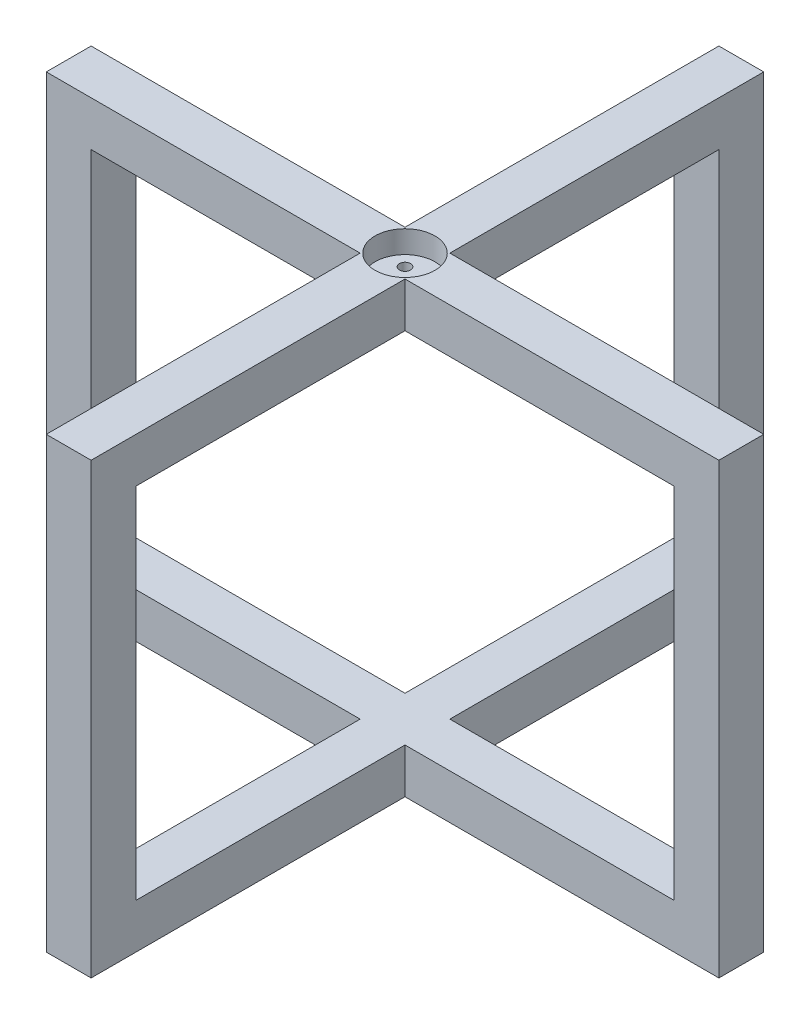
SolidWorks part; units mm, degrees
ref_plane "Front Plane" through (0, 0, 0) normal (0, 0, 1) x (1, 0, 0)
ref_plane "Top Plane" through (0, 0, 0) normal (0, 1, 0) x (1, 0, 0)
ref_plane "Right Plane" through (0, 0, 0) normal (1, 0, 0) x (0, 0, -1)
sketch "Sketch1" plane through (0, 0, 0) normal (0, 0, 1) x (1, 0, 0)
  line L0 (-450, 300) -> (450, 300)
  line L1 (-390, -240) -> (390, -240)
  line L2 (-390, -240) -> (-390, 240)
  line L3 (-390, 240) -> (390, 240)
  line L4 (390, -240) -> (390, 240)
  line L5 (0, 240) -> (0, -240) construction
  line L6 (-390, 0) -> (390, 0) construction
  line L7 (450, -300) -> (450, 300)
  line L8 (-450, -300) -> (450, -300)
  line L9 (-450, -300) -> (-450, 300)
  point P0 (0, 0)
  dimension "D2" = 900
  dimension "D3" = 600
  dimension "D1" = 60
extrude "Boss-Extrude1" add sketch "Sketch1" along normal mid plane 60
sketch "Sketch2" plane through (0, 0, 0) normal (1, 0, 0) x (0, 0, -1)
  line L0 (-450, 300) -> (450, 300)
  line L1 (-390, -240) -> (390, -240)
  line L2 (-390, -240) -> (-390, 240)
  line L3 (-390, 240) -> (390, 240)
  line L4 (390, -240) -> (390, 240)
  line L5 (0, 240) -> (0, -240) construction
  line L6 (-390, 0) -> (390, 0) construction
  line L7 (450, -300) -> (450, 300)
  line L8 (-450, -300) -> (450, -300)
  line L9 (-450, -300) -> (-450, 300)
  point P0 (0, 0)
  dimension "D2" = 900
  dimension "D3" = 600
  dimension "D1" = 60
extrude "Boss-Extrude2" add sketch "Sketch2" along normal mid plane 60
sketch "Sketch3" plane through (0, 300, 0) normal (0, 1, 0) x (1, 0, 0)
  circle A0 centre (0, 0) radius 40
  dimension "D1" = 80
extrude "Cut-Extrude1" cut sketch "Sketch3" against normal blind 30
hole_wizard "Blind dowel hole 0 (size mm)" positions "Sketch4" profile "Sketch5" hole size "Ø1.0" standard "GB"
sketch "Sketch4" plane through (0, 270, 0) normal (0, 1, 0) x (1, 0, 0)
  line L0 (0, 0) -> (-13.5122, 13.5122) construction
  line L2 (0, 0) -> (0, 20.6633) construction
  line L4 (0, 0) -> (5.5395, 5.5395) construction
  point P0 (-14.1421, 14.1421)
  point P2 (14.1421, -14.1421)
  dimension "D1" = 40
  dimension "D2" = 45
  dimension "D3" = 45
sketch "Sketch5" plane through (-14.1421, 270, -14.1421) normal (1, 0, 0) x (0, 0, 1)
  line L0 (0, 0) -> (0, 104.5065)
  line L1 (0, 104.5065) -> (7.5, 100)
  line L2 (7.5, 100) -> (7.5, 0)
  line L5 (7.5, 0) -> (0, 0)
  line L10 (0, 104.5065) -> (-7.5, 100) construction
  line L11 (0, -6.35) -> (0, 107.95) construction
  dimension "孔直径" = 15
  dimension "孔深度" = 100
  dimension "导头角度" = 118
